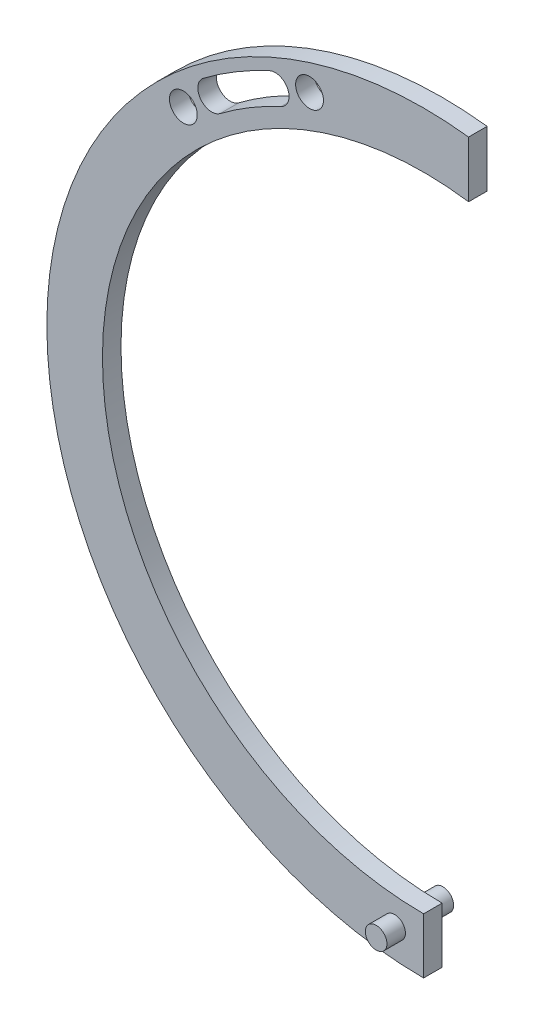
SolidWorks part; units mm, degrees
ref_plane "Front Plane" through (0, 0, 0) normal (0, 0, 1) x (1, 0, 0)
ref_plane "Top Plane" through (0, 0, 0) normal (0, 1, 0) x (1, 0, 0)
ref_plane "Right Plane" through (0, 0, 0) normal (1, 0, 0) x (0, 0, -1)
sketch "Sketch1" plane through (0, 0, 0) normal (0, 0, 1) x (1, 0, 0)
  line L0 (-267.317, 384.5719) -> (-267.3016, 354.3158)
  line L1 (-291.5852, 9.4358) -> (-291.5852, -20.5642)
  arc A1 (-267.317, 384.5719) -> (-291.5852, -20.5642) centre (-291.5852, 182.7307) ccw
  arc A2 (-291.5852, 9.4358) -> (-267.3016, 354.3158) centre (-291.5852, 182.7307) cw
extrude "Boss-Extrude1" add sketch "Sketch1" against normal up to surface (10 mm away)
sketch "Sketch2" plane through (0, 0, 0) normal (0, 0, 1) x (1, 0, 0)
  circle A0 centre (-307.2015, -4.5199) radius 5.8203
extrude "Boss-Extrude2" add sketch "Sketch2" along normal blind 10 and the other way blind 26 contours A0
sketch "Sketch3" plane through (0, 0, 0) normal (0, 0, 1) x (1, 0, 0)
  circle A0 centre (-421.224, 321.6328) radius 7.5
  circle A1 centre (-353.1289, 362.4871) radius 7.5
  arc A2 (-371.6835, 355.0219) -> (-405.9195, 334.4794) centre (-291.5852, 182.7307) ccw construction
  circle A8 centre (-291.5852, 182.7307) radius 190 construction
  arc A9 (-374.8453, 361.8229) -> (-410.4327, 340.4695) centre (-291.5852, 182.7307) ccw
  arc A10 (-368.5217, 348.221) -> (-401.4063, 328.4893) centre (-291.5852, 182.7307) ccw
  arc A11 (-368.5217, 348.221) -> (-374.8453, 361.8229) centre (-371.6835, 355.0219) ccw
  arc A12 (-410.4327, 340.4695) -> (-401.4063, 328.4893) centre (-405.9195, 334.4794) ccw
  point P7 (-389.3426, 345.6524)
  dimension "D1" = 380
  dimension "D2" = 15
  dimension "D3" = 15
  dimension "D5" = 7.5
  dimension "D6" = 40
  dimension "D4" = 80
  dimension "D7" = 20
extrude "Cut-Extrude1" cut sketch "Sketch3" against normal through all both and the other way through all
